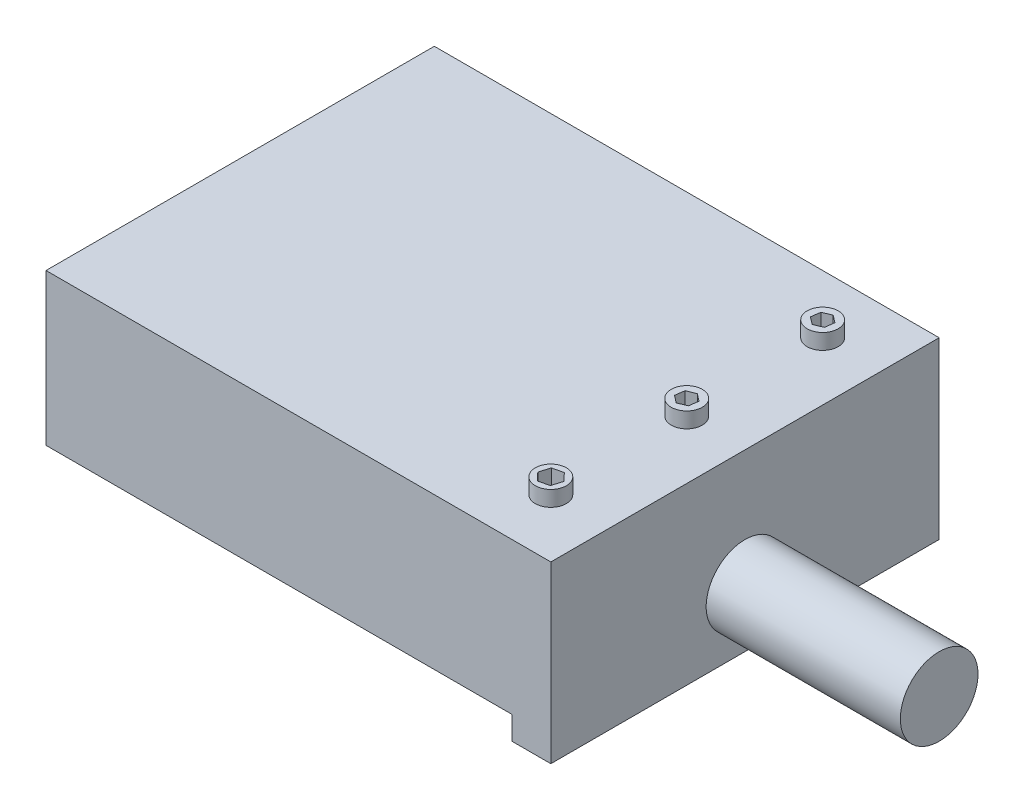
from build123d import *

# Parameters (mm, degrees)
SKETCH1_W           = 70
SKETCH1_H           = 100
BOSS_EXTRUDE1_DEPTH = 30
SKETCH2_R           = 4
BOSS_EXTRUDE2_DEPTH = 4
SKETCH3_R           = 10
BOSS_EXTRUDE3_DEPTH = 50
SKETCH4_W           = 70
SKETCH4_H           = 100
BOSS_EXTRUDE4_DEPTH = 15
CUT_EXTRUDE1_REACH  = 137.577
SKETCH5_W           = 60
SKETCH5_H           = 6
SKETCH6_W           = 100
SKETCH6_H           = 39
BOSS_EXTRUDE5_DEPTH = 60


with BuildPart() as part:
    # Sketch1 → Boss-Extrude1 (new body)
    with BuildSketch(Plane(origin=(0, 0, 0), x_dir=(1, 0, 0), z_dir=(0, 1, 0))):
        Rectangle(SKETCH1_W, SKETCH1_H)
    extrude(amount=BOSS_EXTRUDE1_DEPTH)

    # Sketch2 → Boss-Extrude2 (add)
    # profile 1 of 3: a face of its own
    with BuildSketch(Plane(origin=(0, 30, 0), x_dir=(1, 0, 0), z_dir=(0, 1, 0))):
        with Locations(Location((20, -35, 0), (0, 0, 270))):
            Circle(SKETCH2_R)
        Polygon((21.913058762, -37.035169602), (22.719037957, -34.360827314), (20.805979195, -32.325657712), (18.086941238, -32.964830398), (17.280962043, -35.639172686), (19.194020805, -37.674342288), align=None, mode=Mode.SUBTRACT)
    # profile 2 of 3: a face of its own
    with BuildSketch(Plane(origin=(0, 30, 0), x_dir=(1, 0, 0), z_dir=(0, 1, 0))):
        with Locations(Location((20, 0, 0), (0, 0, 270))):
            Circle(SKETCH2_R)
        Polygon((21.913058762, -1.47020522), (22.229764451, 0.921654877), (20.316705689, 2.391860097), (18.086941238, 1.47020522), (17.770235549, -0.921654877), (19.683294311, -2.391860097), align=None, mode=Mode.SUBTRACT)
    # profile 3 of 3: a face of its own
    with BuildSketch(Plane(origin=(0, 30, 0), x_dir=(1, 0, 0), z_dir=(0, 1, 0))):
        with Locations(Location((20, 35, 0), (0, 0, 270))):
            Circle(SKETCH2_R)
        Polygon((21.913058762, 33.534680981), (22.225532876, 35.924097978), (20.312474114, 37.389416996), (18.086941238, 36.465319019), (17.774467124, 34.075902022), (19.687525886, 32.610583004), align=None, mode=Mode.SUBTRACT)
    extrude(amount=BOSS_EXTRUDE2_DEPTH)

    # Sketch3 → Boss-Extrude3 (add)
    with BuildSketch(Plane(origin=(35, 0, 0), x_dir=(0, 0, -1), z_dir=(1, 0, 0))):
        Circle(SKETCH3_R)
    extrude(amount=BOSS_EXTRUDE3_DEPTH)

    # Sketch4 → Boss-Extrude4 (add)
    with BuildSketch(Plane.XZ):
        Rectangle(SKETCH4_W, SKETCH4_H)
    extrude(amount=BOSS_EXTRUDE4_DEPTH)

    # Sketch5 → Cut-Extrude1 (cut, up to next)
    with BuildSketch(Plane(origin=(0, 0, -50), x_dir=(-1, 0, 0), z_dir=(0, 0, -1)), mode=Mode.PRIVATE) as cut_extrude1_sk1:
        with Locations((5, -12)):
            Rectangle(SKETCH5_W, SKETCH5_H)
    cut_extrude1_tool1 = extrude(cut_extrude1_sk1.sketch, amount=-CUT_EXTRUDE1_REACH, mode=Mode.PRIVATE) & part.part
    add(cut_extrude1_tool1.solids().sort_by_distance((-5, -12, -50))[0], mode=Mode.SUBTRACT)

    # Sketch6 → Boss-Extrude5 (add)
    with BuildSketch(Plane.ZY.offset(35)):
        with Locations((0, 10.5)):
            Rectangle(SKETCH6_W, SKETCH6_H)
    extrude(amount=BOSS_EXTRUDE5_DEPTH)


solid = part.part
